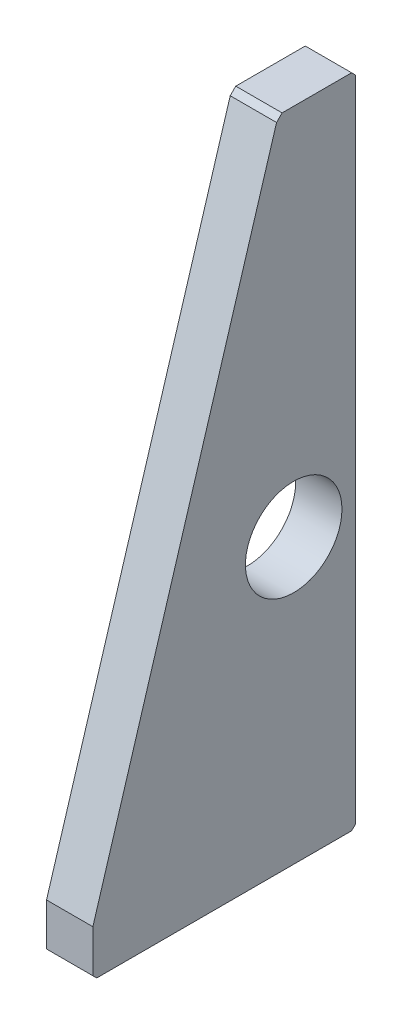
SolidWorks part; units mm, degrees
material "AL6061"
ref_plane "Front Plane" through (0, 0, 0) normal (0, 0, 1) x (1, 0, 0)
ref_plane "Top Plane" through (0, 0, 0) normal (0, 1, 0) x (1, 0, 0)
ref_plane "Right Plane" through (0, 0, 0) normal (1, 0, 0) x (0, 0, -1)
sketch "Sketch1" plane through (0, 0, 0) normal (1, 0, 0) x (0, 0, -1)
  line L0 (0, 0) -> (-68, 0)
  line L1 (-68, 0) -> (-68, 12)
  line L2 (-68, 12) -> (-20, 170)
  line L3 (-20, 170) -> (0, 170)
  line L4 (0, 170) -> (0, 0)
  dimension "D1" = 20
  dimension "D2" = 12
  dimension "D3" = 68
  dimension "D4" = 170
extrude "Boss-Extrude1" add sketch "Sketch1" along normal mid plane 12
hole_wizard "M5 Tapped Hole1" positions "Sketch2" profile "Sketch3" tap size "M5" standard "GB"
sketch "Sketch2" plane through (0, 0, 0) normal (0, 0, -1) x (-1, 0, 0)
  line L0 (0, 0) -> (0, 109.5991) construction
  line L1 (-6, 0) -> (6, 0) construction
  line L2 (-6, 170) -> (6, 170) construction
  point P7 (0, 155)
  point P9 (0, 20)
  dimension "D1" = 20
  dimension "D2" = 15
sketch "Sketch3" plane through (0, 20, 0) normal (1, 0, 0) x (0, 1, 0)
  line L0 (0, 0) -> (0, 13.6618)
  line L1 (0, 13.6618) -> (2.1, 12.4)
  line L2 (2.1, 12.4) -> (2.1, 0)
  line L5 (2.1, 0) -> (0, 0)
  line L10 (0, 13.6618) -> (-2.1, 12.4) construction
  line L11 (0, -6.35) -> (0, 107.95) construction
  dimension "螺纹孔钻头直径" = 4.2
  dimension "螺纹孔钻头深度" = 12.4
  dimension "导头角度" = 118
cosmetic thread "Hole Thread1" parameters "D1"=10, "D2"=5
cosmetic thread "Hole Thread2" parameters "D1"=10, "D2"=5
hole_wizard "M5 Tapped Hole2" positions "Sketch4" profile "Sketch5" tap size "M5" standard "GB"
sketch "Sketch4" plane through (0, 0, 0) normal (0, -1, 0) x (-1, 0, 0)
  line L0 (0, 0) -> (0, -41.4728) construction
  line L1 (-6, -68) -> (6, -68) construction
  line L2 (-6, 0) -> (6, 0) construction
  point P6 (0, -10)
  point P8 (0, -58)
  dimension "D1" = 10
  dimension "D2" = 10
sketch "Sketch5" plane through (0, 0, 58) normal (1, 0, 0) x (0, 0, -1)
  line L0 (0, 0) -> (0, 13.6618)
  line L1 (0, 13.6618) -> (2.1, 12.4)
  line L2 (2.1, 12.4) -> (2.1, 0)
  line L5 (2.1, 0) -> (0, 0)
  line L10 (0, 13.6618) -> (-2.1, 12.4) construction
  line L11 (0, -6.35) -> (0, 107.95) construction
  dimension "螺纹孔钻头直径" = 4.2
  dimension "螺纹孔钻头深度" = 12.4
  dimension "导头角度" = 118
cosmetic thread "Hole Thread3" parameters "D1"=10, "D2"=5
cosmetic thread "Hole Thread4" parameters "D1"=10, "D2"=5
chamfer "Chamfer1" distance 1 angle 45 4 edges at (0, 170, 0) (0, 0, 0) (0, 0, 68) (0, 170, 20)
sketch "Sketch6" plane through (6, 0, 0) normal (1, 0, 0) x (0, 0, -1)
  line L0 (-67, 0) -> (-1, 0) construction
  line L1 (0, 1) -> (0, 169) construction
  circle A0 centre (-16, 73.4) radius 12.5
  dimension "D1" = 73.4
  dimension "D2" = 16
  dimension "D3" = 25
extrude "Cut-Extrude1" cut sketch "Sketch6" against normal through all
